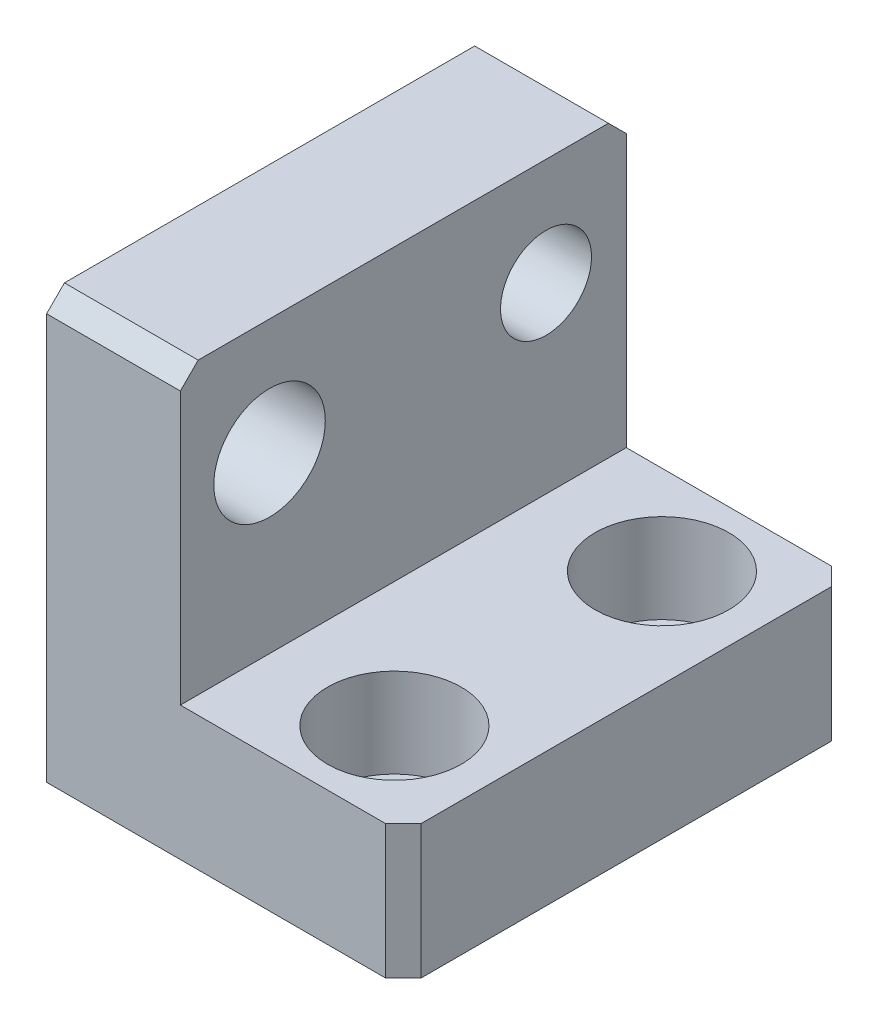
SolidWorks part; units mm, degrees
material "Q235-A"
ref_plane "Front Plane" through (0, 0, 0) normal (0, 0, 1) x (1, 0, 0)
ref_plane "Top Plane" through (0, 0, 0) normal (0, 1, 0) x (1, 0, 0)
ref_plane "Right Plane" through (0, 0, 0) normal (1, 0, 0) x (0, 0, -1)
sketch "Sketch1" plane through (0, 0, 0) normal (0, 0, 1) x (1, 0, 0)
  line L0 (-40.8198, 19.9063) -> (-40.8198, -27.5937)
  line L1 (-40.8198, -27.5937) -> (-0.8198, -27.5937)
  line L2 (-0.8198, -27.5937) -> (-0.8198, -12.5937)
  line L3 (-0.8198, -12.5937) -> (-25.8198, -12.5938)
  line L4 (-25.8198, -12.5938) -> (-25.8198, 19.9063)
  line L5 (-25.8198, 19.9063) -> (-40.8198, 19.9063)
  dimension "D1" = 40
  dimension "D2" = 15
  dimension "D3" = 47.5
  dimension "D4" = 15
extrude "Boss-Extrude1" add sketch "Sketch1" along normal blind 50
sketch "Sketch2" plane through (-25.8198, 0, 0) normal (1, 0, 0) x (0, 0, -1)
  line L0 (-50, -12.5937) -> (-50, 19.9063) construction
  line L2 (0, -12.5937) -> (0, 19.9063) construction
  line L3 (-50, -27.5937) -> (0, -27.5937) construction
  circle A0 centre (-40, 6.9063) radius 3.9167
  circle A1 centre (-9, 7.9063) radius 2.9324
  dimension "D1" = 10
  dimension "D2" = 9
  dimension "D3" = 34.5
  dimension "D4" = 35.5
chamfer "Chamfer2" distance 2 angle 45 4 edges at (-0.8198, -20.0937, 0) (-0.8198, -20.0937, 50) (-33.3198, 19.9063, 0) (-33.3198, 19.9063, 50)
sketch "Sketch10" plane through (0, -12.5937, 0) normal (0, 1, 0) x (1, 0, 0)
  line L0 (-11.8198, -40) -> (-11.8198, -10)
  line L1 (-40.8198, -48) -> (-40.8198, -2) construction
  line L2 (-0.8198, -48) -> (-0.8198, -2) construction
  point P4 (-11.8198, -25)
  point P7 (-0.8198, -25)
  dimension "D1" = 30
  dimension "D2" = 29
  dimension "D3" = 0
hole_wizard "Hole4" positions "Sketch11" profile "Sketch12" legacy end condition through all
sketch "Sketch11" plane through (0, -12.5937, 0) normal (0, 1, 0) x (1, 0, 0)
  point P0 (-11.8198, -10)
  point P3 (-11.8198, -40)
sketch "Sketch12" plane through (-11.8198, -12.5937, 10) normal (1, 0, 0) x (0, 0, 1)
  line L0 (0, 0) -> (0, 15)
  line L1 (0, 15) -> (4.5, 15)
  line L2 (4.5, 15) -> (4.5, 10)
  line L3 (4.5, 10) -> (7.5, 10)
  line L4 (7.5, 10) -> (7.5, 0)
  line L5 (7.5, 0) -> (0, 0)
  line L6 (0, 110) -> (0, -10) construction
  dimension "直径" = 9
  dimension "深度" = 15
  dimension "柱坑直径" = 15
  dimension "柱坑深度" = 10
hole_wizard "M14x1.5 Tapped Hole1" positions "Sketch13" profile "Sketch14" tap size "M14x1.5" standard "GB" end condition through all
sketch "Sketch13" plane through (-25.8198, 0, 0) normal (1, 0, 0) x (0, 0, -1)
  point P0 (-40, 6.9063)
sketch "Sketch14" plane through (-25.8198, 6.9063, 40) normal (0, 1, 0) x (0, 0, -1)
  line L0 (0, 0) -> (0, 15)
  line L1 (0, 15) -> (6.25, 15)
  line L2 (6.25, 15) -> (6.25, 0)
  line L5 (6.25, 0) -> (0, 0)
  line L11 (0, -6.35) -> (0, 107.95) construction
  dimension "通孔螺纹孔钻头直径" = 12.5
  dimension "通孔螺纹孔钻头深度" = 15
cosmetic thread "Cosmetic thread 1" parameters "D2"=14
hole_wizard "M12 Tapped Hole1" positions "Sketch15" profile "Sketch16" tap size "M12" standard "GB" end condition through all
sketch "Sketch15" plane through (-25.8198, 0, 0) normal (1, 0, 0) x (0, 0, -1)
  point P0 (-9, 7.9063)
sketch "Sketch16" plane through (-25.8198, 7.9062, 9) normal (0, 1, 0) x (0, 0, -1)
  line L0 (0, 0) -> (0, 15)
  line L1 (0, 15) -> (5.1, 15)
  line L2 (5.1, 15) -> (5.1, 0)
  line L5 (5.1, 0) -> (0, 0)
  line L11 (0, -6.35) -> (0, 107.95) construction
  dimension "通孔螺纹孔钻头直径" = 10.2
  dimension "通孔螺纹孔钻头深度" = 15
cosmetic thread "Cosmetic thread 2" parameters "D2"=12
